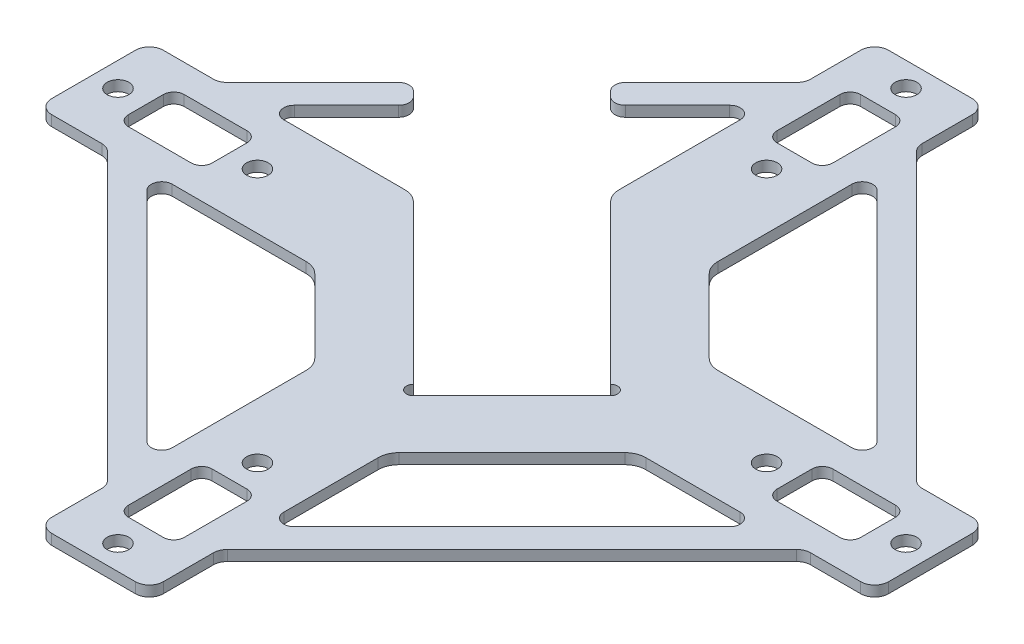
from build123d import *

# Parameters (mm, degrees)
SKETCH_1_R      = 1.55
SKETCH_1_W      = 8
SKETCH_1_H      = 12
SKETCH_1_W_2    = 12
SKETCH_1_H_2    = 8
EXTRUDE_1_DEPTH = 1.5
F_2MM_R         = 2
F_1_5MM_R       = 1.5
F_3MM_R         = 3


with BuildPart() as part:
    # 草图1 → 凸台-拉伸1 (new body)
    with BuildSketch(Plane(origin=(0, 0, 0), x_dir=(1, 0, 0), z_dir=(0, 1, 0))):
        with BuildLine():
            Line((8, 60), (-8, 60))
            Line((-8, 60), (-8, 50))
            Line((-8, 50), (-21.928932188, 36.071067812))
            Line((-21.928932188, 36.071067812), (-19.100505063, 33.242640687))
            Line((-19.100505063, 33.242640687), (-8, 44.343145751))
            Line((-8, 44.343145751), (-8, 22.142135624))
            Line((-8, 22.142135624), (15.556349186, -1.414213562))
            ThreePointArc((15.556349186, -1.414213562), (16.970562748, -1.414213562), (16.970562748, -2.828427125))
            Line((16.970562748, -2.828427125), (2.828427125, -16.970562748))
            ThreePointArc((2.828427125, -16.970562748), (1.414213562, -16.970562748), (1.414213562, -15.556349186))
            Line((1.414213562, -15.556349186), (-22.142135624, 8))
            Line((-22.142135624, 8), (-44.343145751, 8))
            Line((-44.343145751, 8), (-33.242640687, 19.100505063))
            Line((-33.242640687, 19.100505063), (-36.071067812, 21.928932188))
            Line((-36.071067812, 21.928932188), (-50, 8))
            Line((-50, 8), (-60, 8))
            Line((-60, 8), (-60, -8))
            Line((-60, -8), (-50, -8))
            Line((-50, -8), (-8, -50))
            Line((-8, -50), (-8, -60))
            Line((-8, -60), (8, -60))
            Line((8, -60), (8, -50))
            Line((8, -50), (50, -8))
            Line((50, -8), (60, -8))
            Line((60, -8), (60, 8))
            Line((60, 8), (50, 8))
            Line((50, 8), (8, 50))
            Line((8, 50), (8, 60))
        make_face()
        Polygon((-44.343145751, -8), (-20.284271247, -8), (-8, -20.284271247), (-8, -44.343145751), align=None, mode=Mode.SUBTRACT)
        Polygon((8, -44.343145751), (8, -25.941125497), (25.941125497, -8), (44.343145751, -8), align=None, mode=Mode.SUBTRACT)
        Polygon((44.343145751, 8), (20.284271247, 8), (8, 20.284271247), (8, 44.343145751), align=None, mode=Mode.SUBTRACT)
        with Locations(Location((-36.5, 0, 0), (0, 0, 270))):
            Circle(SKETCH_1_R, mode=Mode.SUBTRACT)
        with Locations(Location((0, -56.5, 0), (0, 0, 270))):
            Circle(SKETCH_1_R, mode=Mode.SUBTRACT)
        with Locations((0, -46.5)):
            Rectangle(SKETCH_1_W, SKETCH_1_H, mode=Mode.SUBTRACT)
        with Locations(Location((0, -36.5, 0), (0, 0, 270))):
            Circle(SKETCH_1_R, mode=Mode.SUBTRACT)
        with Locations(Location((-56.5, 0, 0), (0, 0, 270))):
            Circle(SKETCH_1_R, mode=Mode.SUBTRACT)
        with Locations((-46.5, 0)):
            Rectangle(SKETCH_1_W_2, SKETCH_1_H_2, mode=Mode.SUBTRACT)
        with Locations(Location((36.5, 0, 0), (0, 0, 270))):
            Circle(SKETCH_1_R, mode=Mode.SUBTRACT)
        with Locations((46.5, 0)):
            Rectangle(SKETCH_1_W_2, SKETCH_1_H_2, mode=Mode.SUBTRACT)
        with Locations(Location((56.5, 0, 0), (0, 0, 270))):
            Circle(SKETCH_1_R, mode=Mode.SUBTRACT)
        with Locations(Location((0, 36.5, 0), (0, 0, 270))):
            Circle(SKETCH_1_R, mode=Mode.SUBTRACT)
        with Locations((0, 46.5)):
            Rectangle(SKETCH_1_W, SKETCH_1_H, mode=Mode.SUBTRACT)
        with Locations(Location((0, 56.5, 0), (0, 0, 270))):
            Circle(SKETCH_1_R, mode=Mode.SUBTRACT)
    extrude(amount=EXTRUDE_1_DEPTH)

    # 2mm
    f_2mm_edges = [part.edges().sort_by_distance(p)[0] for p in [
        (-60, 0.75, 8),
        (-60, 0.75, -8),
        (-50, 0.75, -8),
        (-8, 0.75, -50),
        (-8, 0.75, -60),
        (8, 0.75, -60),
        (8, 0.75, -50),
        (50, 0.75, -8),
        (60, 0.75, -8),
        (60, 0.75, 8),
        (50, 0.75, 8),
        (8, 0.75, 50),
        (8, 0.75, 60),
        (-8, 0.75, 60),
        (-8, 0.75, 50),
        (-50, 0.75, 8),
    ]]
    fillet(f_2mm_edges, radius=F_2MM_R)

    # 1.5mm
    f_1_5mm_edges = [part.edges().sort_by_distance(p)[0] for p in [
        (-4, 0.75, 52.5),
        (4, 0.75, 52.5),
        (4, 0.75, 40.5),
        (-4, 0.75, 40.5),
        (52.5, 0.75, 4),
        (52.5, 0.75, -4),
        (40.5, 0.75, -4),
        (40.5, 0.75, 4),
        (4, 0.75, -52.5),
        (-4, 0.75, -52.5),
        (-4, 0.75, -40.5),
        (4, 0.75, -40.5),
        (-52.5, 0.75, -4),
        (-52.5, 0.75, 4),
        (-40.5, 0.75, 4),
        (-40.5, 0.75, -4),
        (8, 0.75, -44.343145751),
        (44.343145751, 0.75, -8),
        (44.343145751, 0.75, 8),
        (8, 0.75, 44.343145751),
        (-36.071067812, 0.75, -21.928932188),
        (-33.242640687, 0.75, -19.100505063),
        (-44.343145751, 0.75, -8),
        (-8, 0.75, -44.343145751),
        (-19.100505063, 0.75, -33.242640687),
        (-21.928932188, 0.75, -36.071067812),
        (-8, 0.75, 44.343145751),
        (-44.343145751, 0.75, 8),
    ]]
    fillet(f_1_5mm_edges, radius=F_1_5MM_R)

    # 3mm
    f_3mm_edges = [part.edges().sort_by_distance(p)[0] for p in [
        (8, 0.75, -20.284271247),
        (20.284271247, 0.75, -8),
        (25.941125497, 0.75, 8),
        (8, 0.75, 25.941125497),
        (-22.142135624, 0.75, -8),
        (-8, 0.75, -22.142135624),
        (-8, 0.75, 20.284271247),
        (-20.284271247, 0.75, 8),
    ]]
    fillet(f_3mm_edges, radius=F_3MM_R)


solid = part.part
